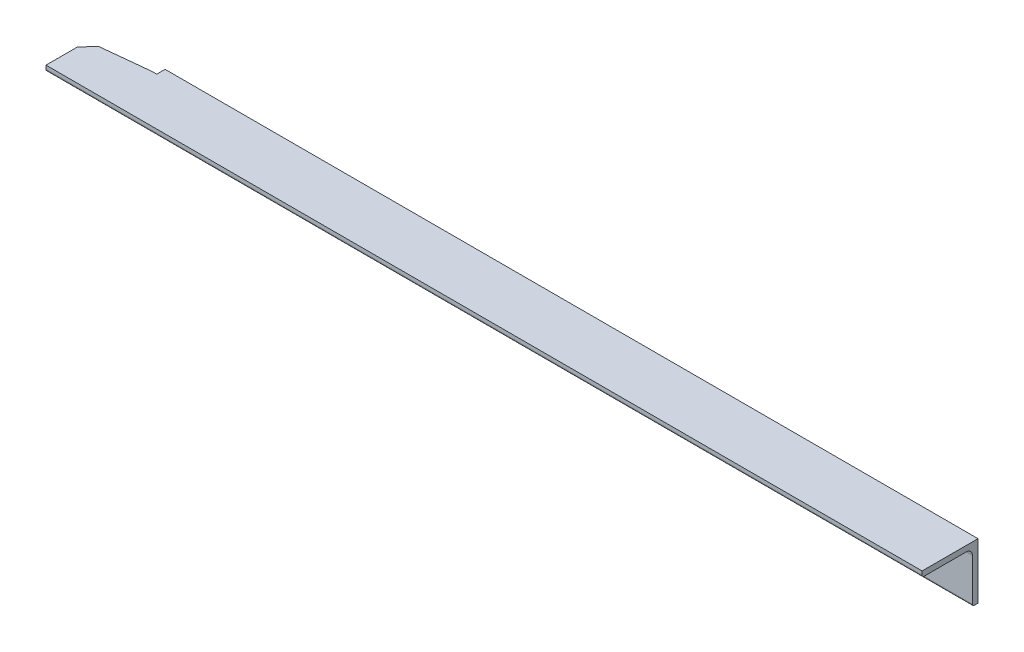
from build123d import *

# Parameters (mm, degrees)
GBT706_2008_050_5_1_DEPTH = 783.5
CUT_EXTRUDE_1_DEPTH       = 399.080472392


with BuildPart() as part:
    # Sketch1 → Gbt706-2008 热轧等边角钢 050×5(1) (new body)
    with BuildSketch(Plane(origin=(391.75, 0, 0), x_dir=(0, -1, 0), z_dir=(-1, 0, 0))):
        with BuildLine():
            Line((0, 0), (0, 50))
            Line((0, 50), (3.333333333, 50))
            ThreePointArc((3.333333333, 50), (4.511844635, 49.511844635), (5, 48.333333333))
            Line((5, 48.333333333), (5, 10.5))
            ThreePointArc((5, 10.5), (6.610912703, 6.610912703), (10.5, 5))
            Line((10.5, 5), (48.333333333, 5))
            ThreePointArc((48.333333333, 5), (49.511844635, 4.511844635), (50, 3.333333333))
            Line((50, 3.333333333), (50, 0))
            Line((50, 0), (0, 0))
        make_face()
    extrude(amount=GBT706_2008_050_5_1_DEPTH)

    # 草图2 → 切除-拉伸1 (cut, through all)
    with BuildSketch(Plane(origin=(0, 0, 0), x_dir=(1, 0, 0), z_dir=(0, 1, 0))):
        Polygon((-335.25, 0), (-335.25, -7.501394609), (-339.727357684, -7.501394609), (-382.795284633, -12.028016136), (-391.75, -21.973235089), (-391.75, -52.501394609), (-406.75, -52.501394609), (-406.75, 7.498605391), (-335.25, 7.498605391), align=None)
    extrude(amount=-CUT_EXTRUDE_1_DEPTH, mode=Mode.SUBTRACT)


solid = part.part
